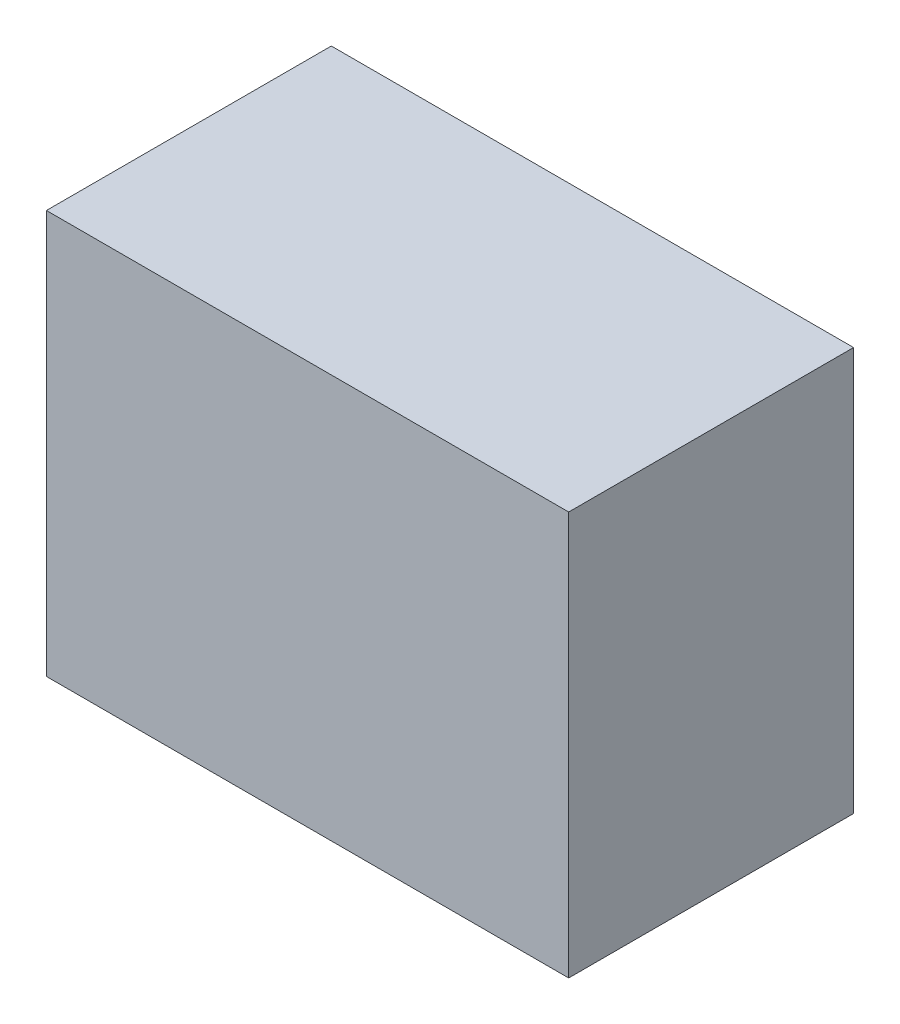
from build123d import *

# Parameters (mm, degrees)
SKETCH1_W           = 1100
SKETCH1_H           = 850
BOSS_EXTRUDE1_DEPTH = 600


with BuildPart() as part:
    # Sketch1 → Boss-Extrude1 (new body)
    with BuildSketch(Plane.XY):
        with Locations((550, 425)):
            Rectangle(SKETCH1_W, SKETCH1_H)
    extrude(amount=BOSS_EXTRUDE1_DEPTH)


solid = part.part
